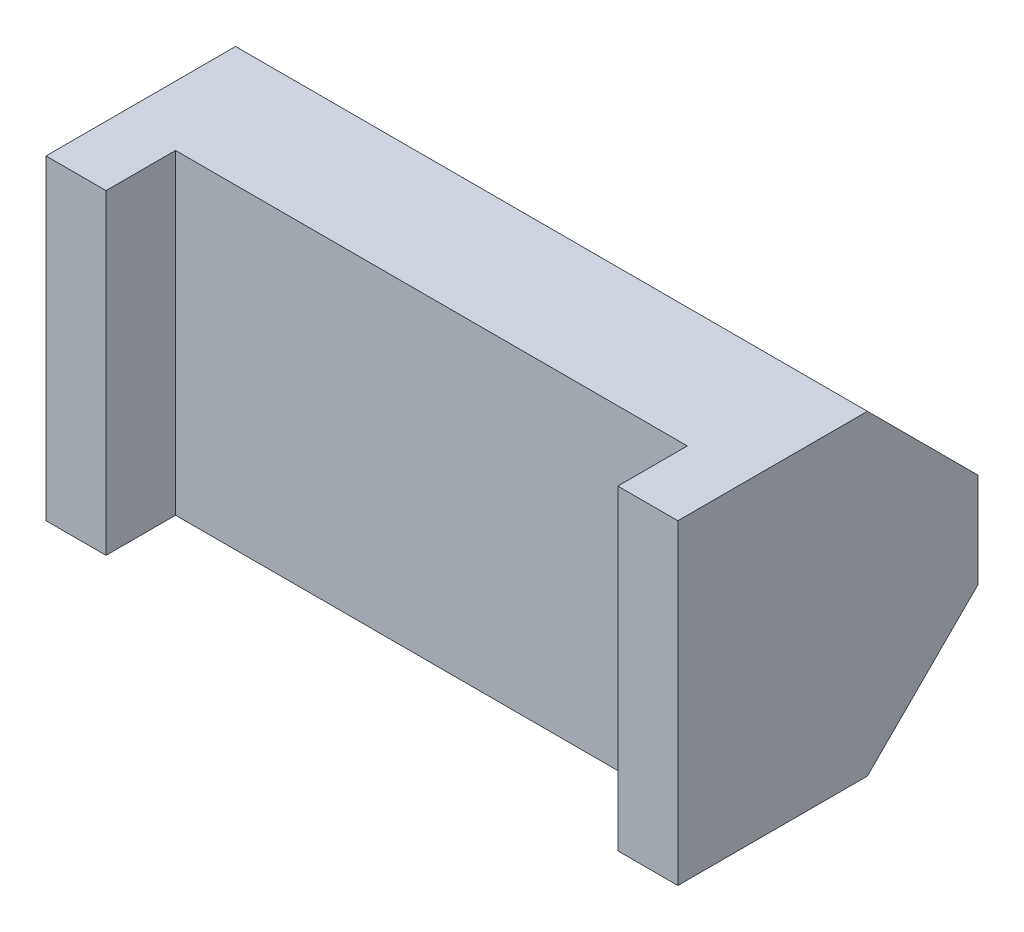
from build123d import *

# Parameters (mm, degrees)
SKETCH_1_W          = 20
SKETCH_1_H          = 10
EXTRUDE_1_DEPTH     = 9.5
SKETCH_2_W          = 16.2
SKETCH_2_H          = 29.89512134
CUT_EXTRUDE_1_DEPTH = 2.2
CUT_EXTRUDE_2_DEPTH = 23.699118926


with BuildPart() as part:
    # 草图1 → 凸台-拉伸1 (new body)
    with BuildSketch(Plane.XY):
        Rectangle(SKETCH_1_W, SKETCH_1_H)
    extrude(amount=EXTRUDE_1_DEPTH)

    # 草图2 → 切除-拉伸1 (cut)
    with BuildSketch(Plane.XY.offset(9.5)):
        Rectangle(SKETCH_2_W, SKETCH_2_H)
    extrude(amount=-CUT_EXTRUDE_1_DEPTH, mode=Mode.SUBTRACT)

    # 草图3 → 切除-拉伸2 (cut, through all)
    with BuildSketch(Plane.ZY.offset(10)):
        Polygon((0, 5), (3.5, 5), (0, 1.5), align=None)
    cut_extrude_2 = extrude(amount=-CUT_EXTRUDE_2_DEPTH, mode=Mode.SUBTRACT)

    # 镜向1: 切除-拉伸2 across plane
    add(cut_extrude_2.mirror(Plane.ZX), mode=Mode.SUBTRACT)


solid = part.part
